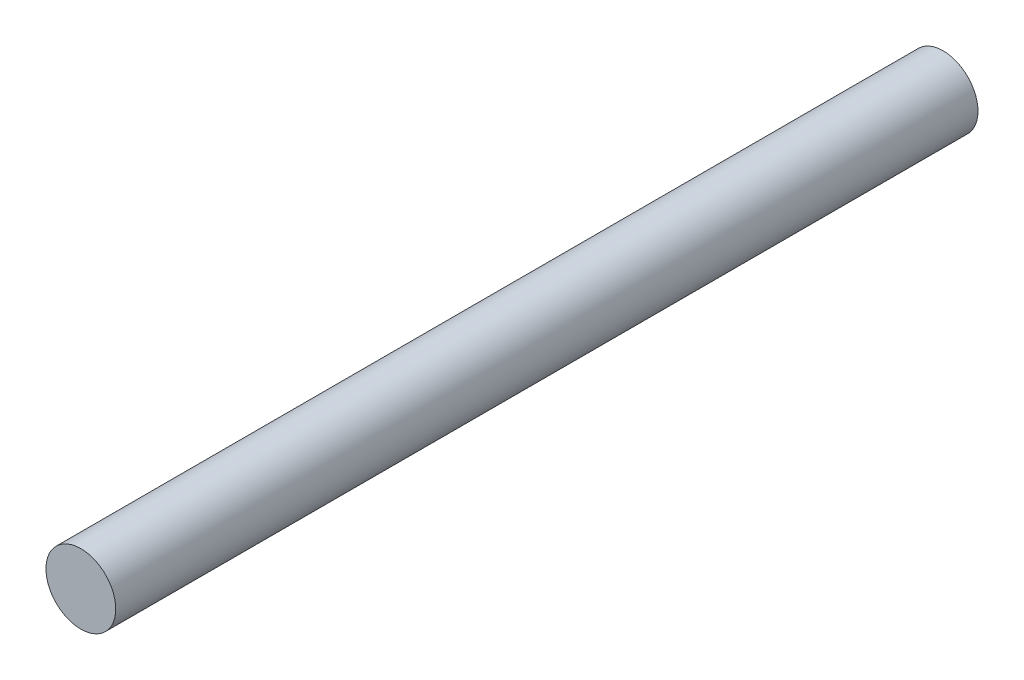
from build123d import *

# Parameters (mm, degrees)
SKETCH_1_R      = 8.5
EXTRUDE_1_DEPTH = 210


with BuildPart() as part:
    # 草图1 → 凸台-拉伸1 (new body)
    with BuildSketch(Plane.XY):
        Circle(SKETCH_1_R)
    extrude(amount=EXTRUDE_1_DEPTH)


solid = part.part
